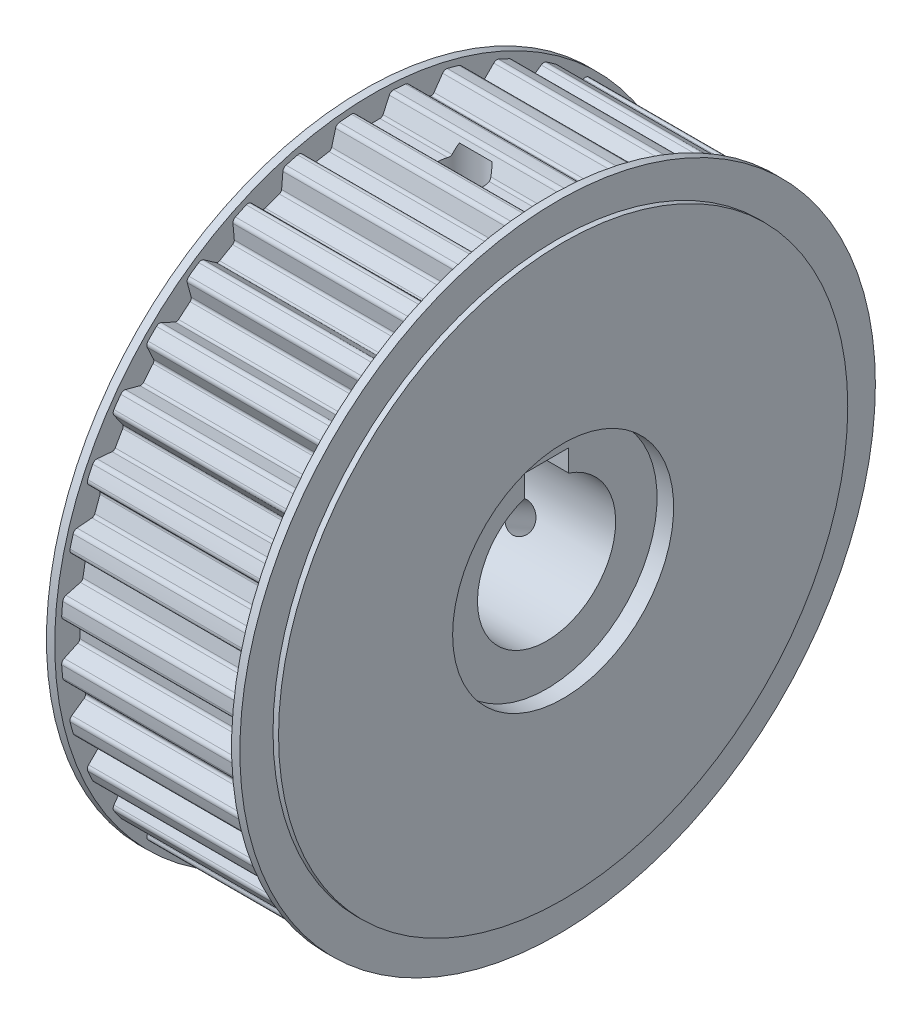
SolidWorks part; units mm, degrees
material "6061 合金"
ref_plane "前视" through (0, 0, 0) normal (0, 0, 1) x (1, 0, 0)
ref_plane "上视" through (0, 0, 0) normal (0, 1, 0) x (1, 0, 0)
ref_plane "右视" through (0, 0, 0) normal (1, 0, 0) x (0, 0, -1)
sketch "草图1" plane through (0, 0, 0) normal (1, 0, 0) x (0, 0, -1)
  line L0 (0, 56.37) -> (0, 56.751) construction
  circle A1 centre (0, 0) radius 56.37
  circle A2 centre (0, 0) radius 56.751 construction
  dimension "D2" = 112.74
  dimension "D3" = 0.381
extrude "拉伸1" add sketch "草图1" along normal mid plane 32
sketch "草图2" plane through (16, 0, 0) normal (1, 0, 0) x (0, 0, -1)
  line L0 (0, 0) -> (0, 61.5267) construction
  line L1 (-3.285, 56.2742) -> (-1.7442, 52.97)
  line L2 (-1.7442, 52.97) -> (1.7442, 52.97)
  line L3 (1.7442, 52.97) -> (3.285, 56.2742)
  circle A0 centre (0, 0) radius 56.37 construction
  arc A1 (3.285, 56.2742) -> (-3.285, 56.2742) centre (0, 0) ccw
  dimension "D2" = 3.4
  dimension "D3" = 25
  dimension "D1" = 6.57
extrude "拉伸2" cut sketch "草图2" against normal up to surface (32 mm away) up to face at (-16, 0, -56.37)
fillet "圆角1" radius 0.6 2 edges at (0, 52.97, -1.7442) (0, 52.97, 1.7442)
fillet "圆角2" radius 0.8 2 edges at (0, 56.2742, -3.285) (0, 56.2742, 3.285)
pattern_circular "阵列(圆周)1" count 36 over 360 about axis through (0, 0, 0) along (1, 0, 0) of "拉伸2", "圆角1", "圆角2"
sketch "草图6" plane through (16, 0, 0) normal (1, 0, 0) x (0, 0, -1)
  circle A0 centre (0, 0) radius 57.5
  dimension "D1" = 115
extrude "凸台-拉伸2" add sketch "草图6" along normal blind 1.5
sketch "草图7" plane through (17.5, 0, 0) normal (1, 0, 0) x (0, 0, -1)
  circle A0 centre (0, 0) radius 51.5
  dimension "D1" = 103
extrude "凸台-拉伸3" add sketch "草图7" along normal blind 1
mirror "镜向2" about plane through (0, 0, 0) normal (1, 0, 0) of "凸台-拉伸3", "凸台-拉伸2"
sketch "草图8" plane through (-18.5, 0, 0) normal (-1, 0, 0) x (0, 0, 1)
  circle A0 centre (0, 0) radius 12.5
  dimension "D1" = 25
extrude "切除-拉伸1" cut sketch "草图8" against normal through all
sketch "草图9" plane through (-18.5, 0, 0) normal (-1, 0, 0) x (0, 0, 1)
  circle A0 centre (0, 0) radius 23.5
  dimension "D1" = 47
extrude "切除-拉伸2" [suppressed] cut sketch "草图9" against normal blind 32.5
sketch "草图10" [suppressed] plane through (0, 0, 0) normal (0, 1, 0) x (1, 0, 0)
  line L0 (14, 23.5) -> (-18.5, 23.5) construction
  line L1 (-15.8, 23.5) -> (-14, 23.5)
  line L2 (-15.8, 23.5) -> (-15.8, 24.5)
  line L3 (-15.8, 24.5) -> (-14, 24.5)
  line L4 (-14, 23.5) -> (-14, 24.5)
  line L5 (14, 23.5) -> (14, -23.5) construction
  line L6 (0, 0) -> (-33.3455, 0) construction
  dimension "D1" = 1.8
  dimension "D2" = 28
  dimension "D3" = 24.5
revolve "切除-旋转1" [suppressed] cut sketch "草图10" angle 360 about L6
sketch "草图11" plane through (-18.5, 0, 0) normal (-1, 0, 0) x (0, 0, 1)
  circle A0 centre (0, 0) radius 20
  dimension "D1" = 40
extrude "切除-拉伸3" cut sketch "草图11" against normal blind 3
mirror "镜向3" about plane through (0, 0, 0) normal (1, 0, 0) of "切除-拉伸3"
sketch "草图12" plane through (-18.5, 0, 0) normal (-1, 0, 0) x (0, 0, 1)
  line L0 (0, 0) -> (0, 17.6786) construction
  line L1 (-4, 15.8) -> (4, 15.8)
  line L2 (-4, 15.8) -> (-4, 10.1071)
  line L3 (-4, 10.1071) -> (4, 10.1071)
  line L4 (4, 15.8) -> (4, 10.1071)
  line L5 (0, 0) -> (24.8621, 0) construction
  circle A0 centre (0, 0) radius 12.5 construction
  dimension "D1" = 8
  dimension "D2" = 28.3
extrude "切除-拉伸4" cut sketch "草图12" against normal through all
ref_plane "基准面1" through (0, 55, 0) normal (0, 1, 0) x (1, 0, 0)
hole_wizard "M6 螺纹孔1" positions "草图14" profile "草图13" tap size "M6" standard "Gb"
sketch "草图14" plane through (0, 55, 0) normal (0, 1, 0) x (1, 0, 0)
  point P0 (0, 0)
cosmetic thread "孔螺蚊线1" parameters "D1"=12, "D2"=6
sketch "草图13" plane through (0, 55, 0) normal (1, 0, 0) x (0, 0, 1)
  line L0 (0, 0) -> (0, 51.5022)
  line L1 (0, 51.5022) -> (2.5, 50)
  line L2 (2.5, 50) -> (2.5, 0)
  line L5 (2.5, 0) -> (0, 0)
  line L10 (0, 51.5022) -> (-2.5, 50) construction
  line L11 (0, -6.35) -> (0, 107.95) construction
  dimension "螺纹孔钻头直径" = 5
  dimension "螺纹孔钻头深度" = 50
  dimension "导头角度" = 118
sketch "草图15" plane through (0, 55, 0) normal (0, 1, 0) x (1, 0, 0)
  circle A0 centre (0, 0) radius 4
  dimension "D1" = 8
extrude "切除-拉伸5" cut sketch "草图15" against normal blind 30
pattern_circular "阵列(圆周)2" count 2 over 120 about axis through (18.5, 0, 0) along (-1, 0, 0) of "切除-拉伸5", "M6 螺纹孔1"
